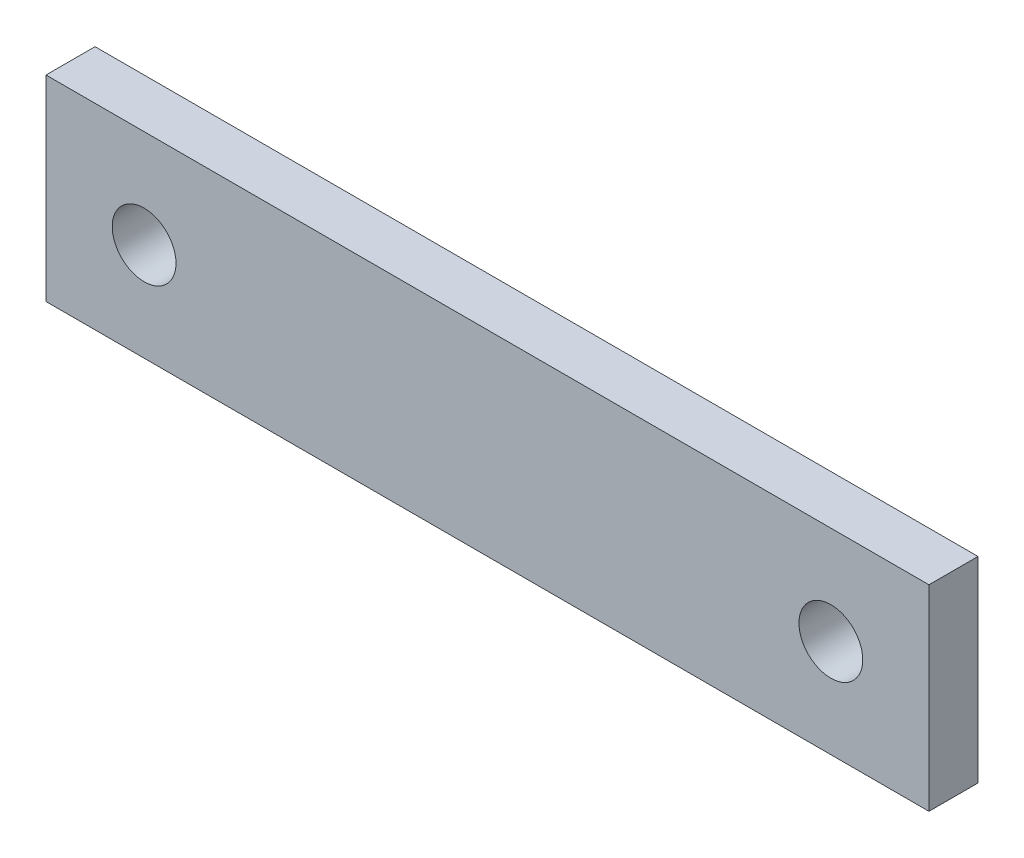
SolidWorks part; units mm, degrees
material "Q235B"
ref_plane "Front Plane" through (0, 0, 0) normal (0, 0, 1) x (1, 0, 0)
ref_plane "Top Plane" through (0, 0, 0) normal (0, 1, 0) x (1, 0, 0)
ref_plane "Right Plane" through (0, 0, 0) normal (1, 0, 0) x (0, 0, -1)
sketch "Sketch1" plane through (0, 0, 0) normal (0, 0, 1) x (1, 0, 0)
  line L1 (90, -20) -> (-90, -20)
  line L2 (90, -20) -> (90, 20)
  line L3 (90, 20) -> (-90, 20)
  line L4 (-90, -20) -> (-90, 20)
  line L5 (90, -20) -> (-90, 20) construction
  line L6 (90, 20) -> (-90, -20) construction
  point P0 (0, 0)
  dimension "D1" = 40
  dimension "D2" = 180
extrude "Boss-Extrude1" add sketch "Sketch1" along normal mid plane 10
hole_wizard "Ø13.0 (13) Diameter Hole1" positions "Sketch2" profile "Sketch3" hole size "Ø13.0" standard "GB" end condition through all
sketch "Sketch2" plane through (0, 0, 5) normal (0, 0, 1) x (1, 0, 0)
  line L0 (0, 20) -> (0, 0) construction
  line L1 (90, 20) -> (-90, 20) construction
  point P0 (-70, 0)
  point P12 (70, 0)
  dimension "D1" = 140
  dimension "D3" = 20
sketch "Sketch3" plane through (-70, 0, 5) normal (1, 0, 0) x (0, -1, 0)
  line L0 (0, 0) -> (0, 10)
  line L1 (0, 10) -> (6.5, 10)
  line L2 (6.5, 10) -> (6.5, 0)
  line L5 (6.5, 0) -> (0, 0)
  line L11 (0, -6.35) -> (0, 107.95) construction
  dimension "通孔孔直径" = 13
  dimension "通孔孔深度" = 10
hole_wizard "M8 Tapped Hole1" positions "Sketch4" profile "Sketch5" tap size "M8" standard "GB"
sketch "Sketch4" plane through (0, 0, 6) normal (0, 0, 1) x (1, 0, 0)
  line L0 (60, 235) -> (-60, 235) construction
  line L1 (0, 200) -> (0, 120) construction
  point P0 (0, 200)
  point P11 (0, 120)
  point P12 (0, 40)
  point P13 (0, -40)
  point P14 (0, -120)
  point P15 (0, -200)
  dimension "D1" = 35
  dimension "D3" = 80
  dimension "D2" = 6
sketch "Sketch5" plane through (0, 200, 6) normal (1, 0, 0) x (0, -1, 0)
  line L0 (0, 0) -> (0, 12)
  line L1 (0, 12) -> (3.4, 12)
  line L2 (3.4, 12) -> (3.4, 0)
  line L5 (3.4, 0) -> (0, 0)
  line L11 (0, -6.35) -> (0, 107.95) construction
  dimension "通孔螺纹孔钻头直径" = 6.8
  dimension "通孔螺纹孔钻头深度" = 12
cosmetic thread "Cosmetic Thread1" [suppressed] parameters "D2"=8
cosmetic thread "Cosmetic Thread2" [suppressed] parameters "D2"=8
cosmetic thread "Cosmetic Thread3" [suppressed] parameters "D2"=8
cosmetic thread "Cosmetic Thread4" [suppressed] parameters "D2"=8
cosmetic thread "Cosmetic Thread5" [suppressed] parameters "D2"=8
cosmetic thread "Cosmetic Thread6" [suppressed] parameters "D2"=8
